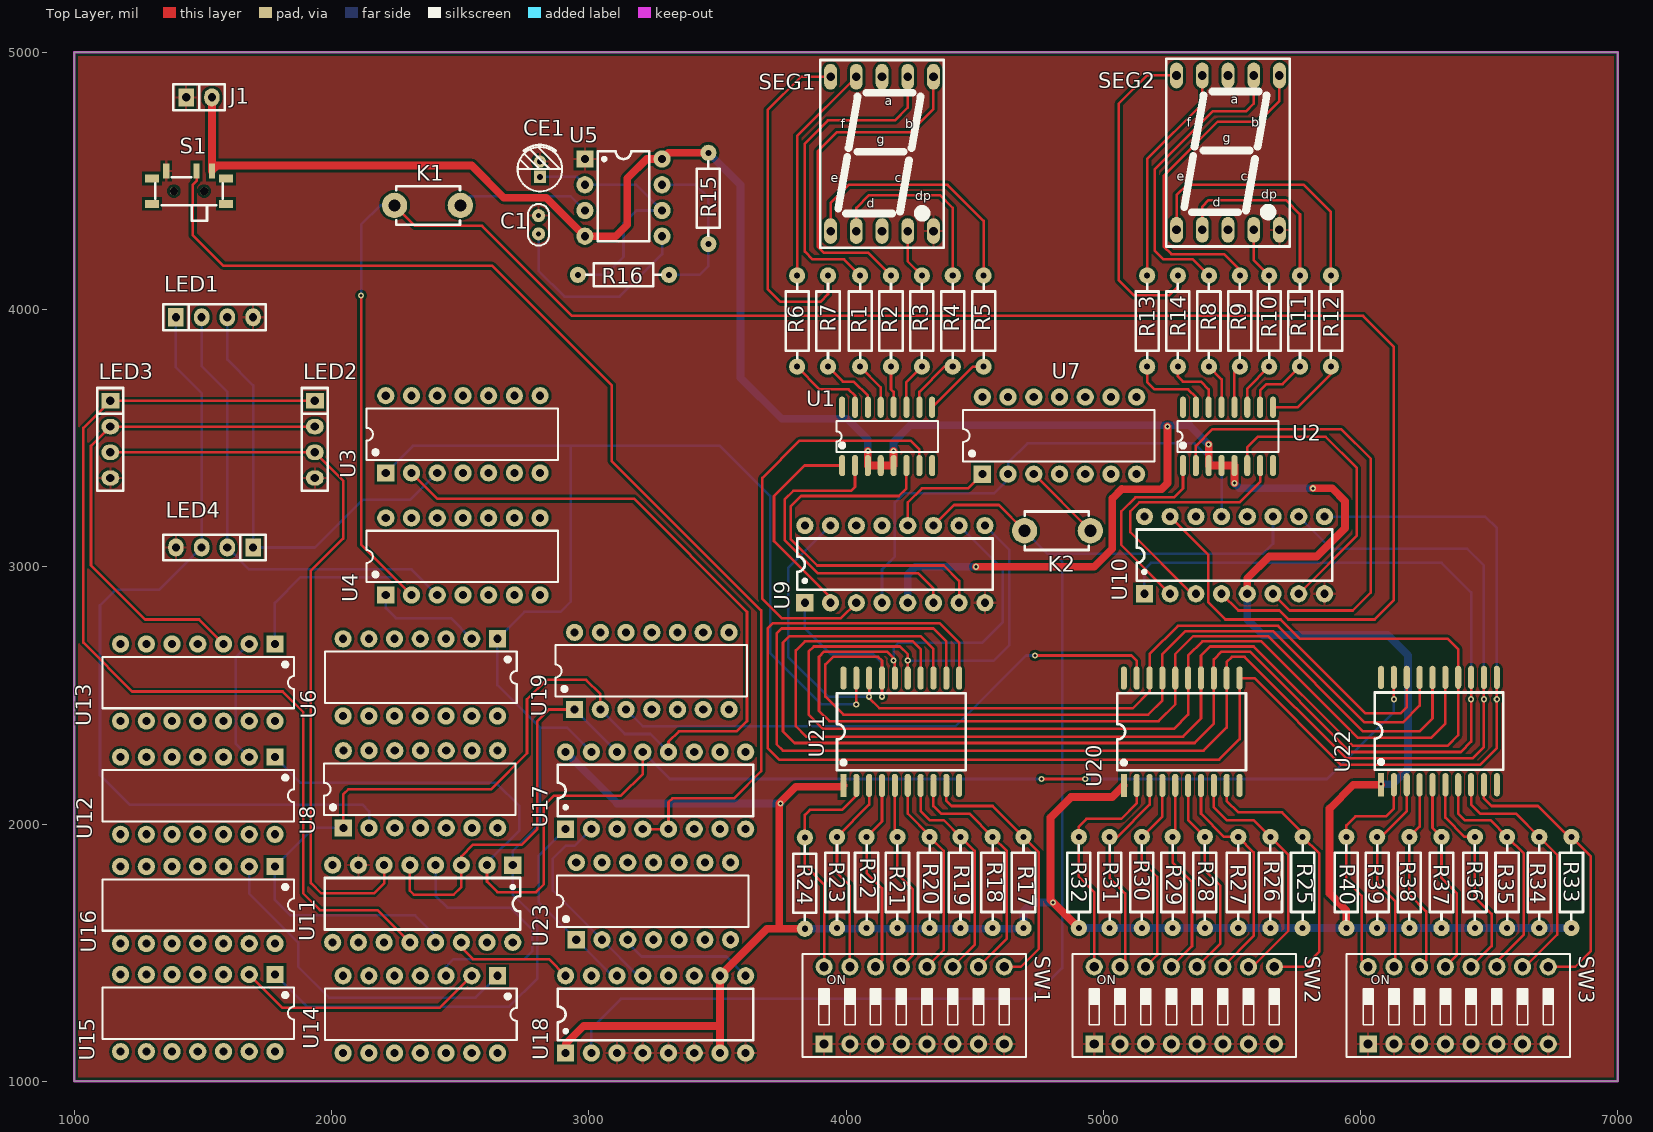
[diagram p0: Top Layer view]
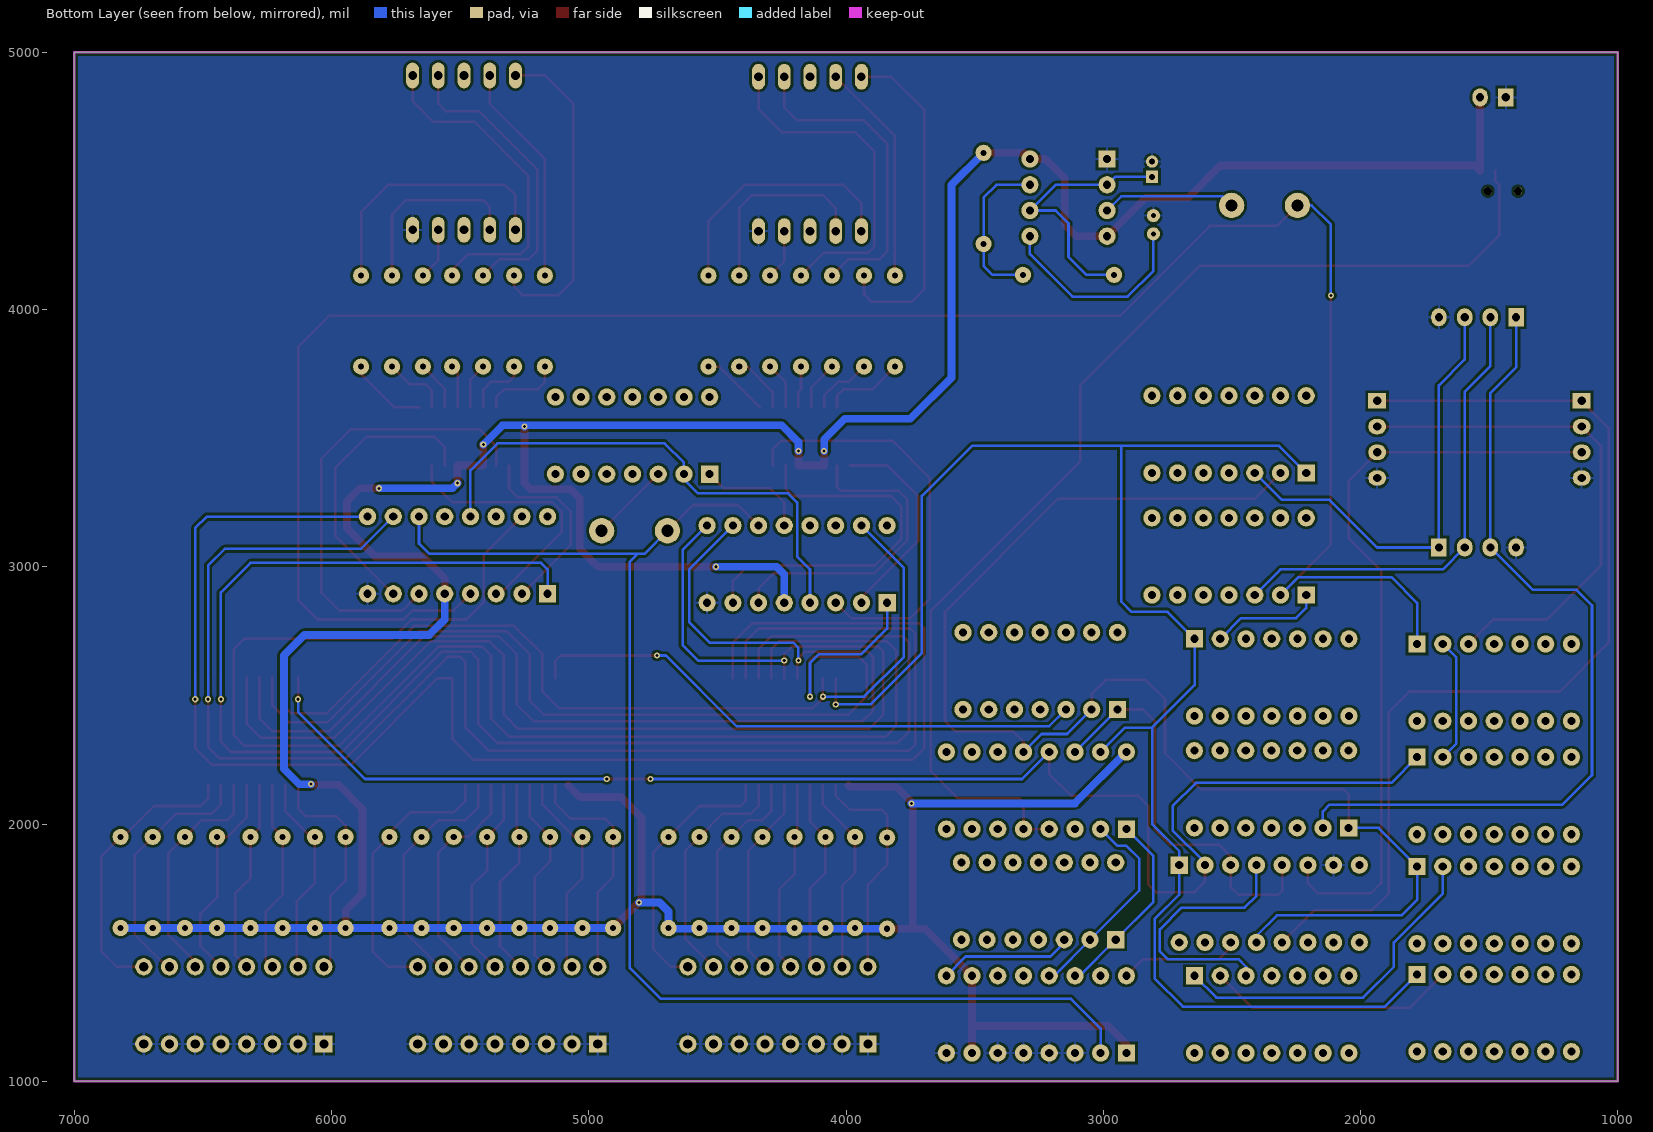
[diagram p1: Bottom Layer view, seen from below]
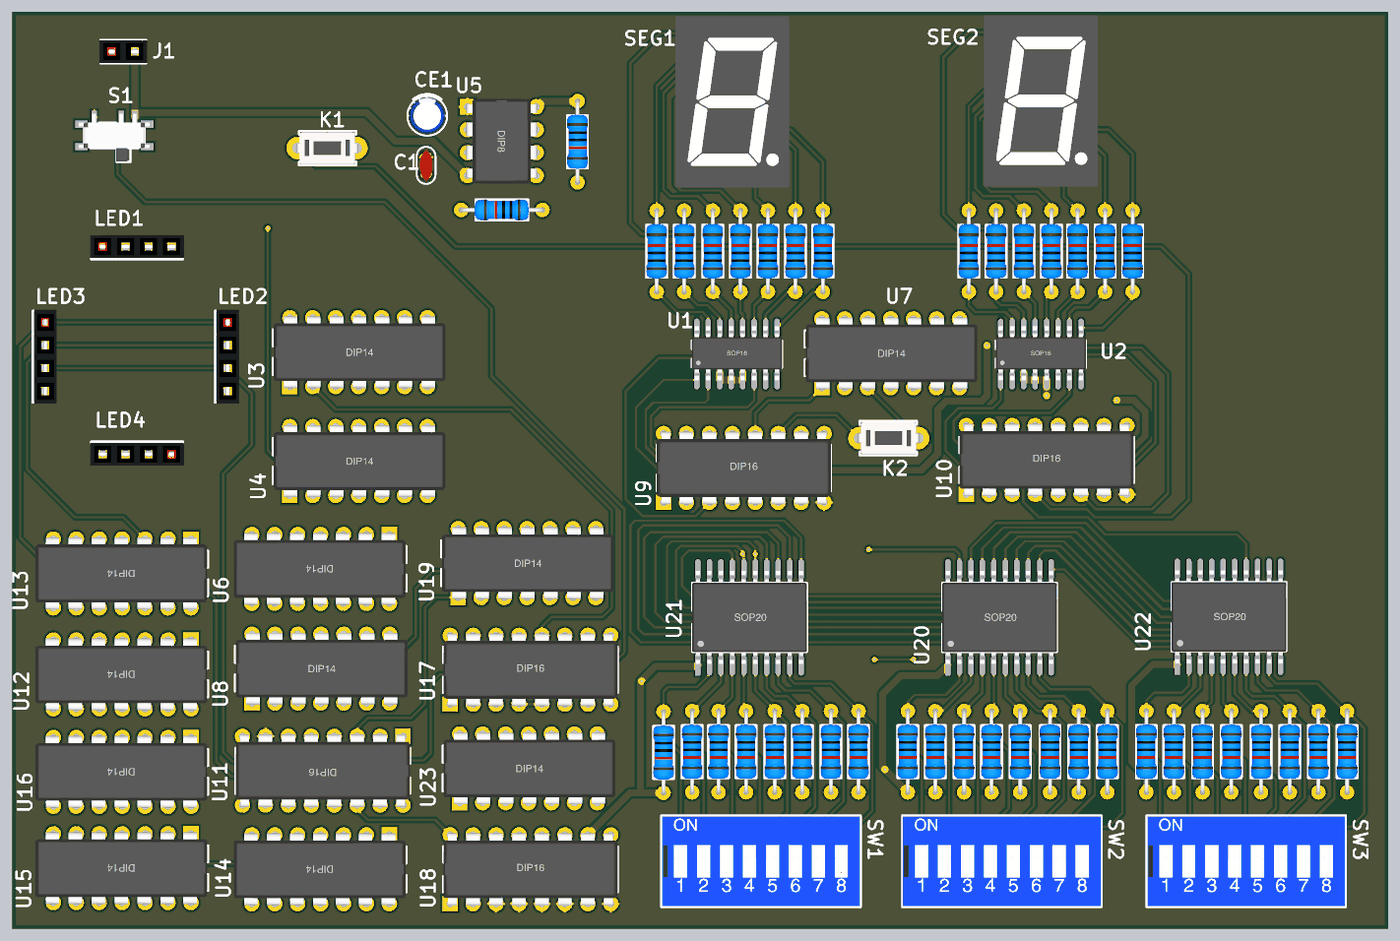
[diagram p2: 3D render of the assembled board from above, using the file's embedded part models]
# Altium PCB MISC82158.PcbDoc
Units mil, origin at the board's own origin, x right, y up, seen from the top; angles counter-clockwise.
Board outline 6000 x 4000 mil, 2 copper layers (Top Layer, Bottom Layer); 78 components, 100 nets, 531 pads, 23 vias.

## Layer stack, top to bottom (the 12.6 mil dielectric is the usual default, probably not edited)
Top Solder: solder mask 0.4, Solder Resist, Dk 3.5
Top Layer: signal copper 1.4
Dielectric 1: dielectric 12.6, FR-4, Dk 4.8
Bottom Layer: signal copper 1.4
Bottom Solder: solder mask 0.4, Solder Resist, Dk 3.5

## Board outline
1000,1000 7000,1000 7000,5000 1000,5000

## Design rules (kind name [scope] priority, off if disabled: settings)
Clearance [All] p1: gap=10
HoleSize [All] p1: absolutevalues=TRUE maxlimit=10000 minlimit=1 maxpercent=80.000 minpercent=20.000
MinimumSolderMaskSliver [All] p1: minsoldermaskwidth=0
PolygonConnect [All] p1: connectstyle=Relief reliefconductorwidth=10 reliefentries=4 polygonreliefangle="90 Angle" airgapwidth=10
RoutingVias [All] p1: holewidth=28 width=50 viastyle="Through Hole" minholewidth=28 minwidth=50 maxholewidth=28 maxwidth=50
SilkToSilkClearance [All] p1: silktosilkclearance=0
SilkToSolderMaskClearance [IsPad] p1: minsilkscreentomaskgap=0 clearancetoexposedcopper=TRUE
SolderMaskExpansion [All] p1: expansion=4
Width [All] p1: maxlimit=100 minlimit=10 preferedwidth=10
26 further rules are at their usual default settings.

## Components (designator, comment, footprint, x,y, rotation, side; value= is the part's Value field where it differs from the comment)
C1 "10nF" "CC 1.8*3.6" 2805,4329.57 r270 top
CE1 "10uF" "CAP 1.5*4*8" 2810,4545.47 r90 top
J1 "Female HDR1X2" Fe-HDR1X2/2.54-S 1435,4825 r0 top
K1 "KEY" DIP-3X6X4.3 2245,4405 r0 top
K2 "KEY" DIP-3X6X4.3 4950,3140 r180 top
LED1 "RGB-3528" Fe-HDR1X4/2.54-S 1395,3970 r90 top
LED2 "RGB-3528" Fe-HDR1X4/2.54-S 1935,3645 r0 top
LED3 "RGB-3528" Fe-HDR1X4/2.54-S 1140,3645 r0 top
LED4 "RGB-3528" Fe-HDR1X4/2.54-S 1695,3075 r270 top
R1 "200" "RS 1/4W" 4055,3955 r90 top
R2 "200" "RS 1/4W" 4175,3955 r90 top
R3 "200" "RS 1/4W" 4295,3955 r90 top
R4 "200" "RS 1/4W" 4415,3955 r90 top
R5 "200" "RS 1/4W" 4535,3955 r90 top
R6 "200" "RS 1/4W" 3810,3955 r90 top
R7 "200" "RS 1/4W" 3930,3955 r90 top
R8 "200" "RS 1/4W" 5410.92,3955 r90 top
R9 "200" "RS 1/4W" 5530.92,3955 r90 top
R10 "200" "RS 1/4W" 5645,3955 r90 top
R11 "200" "RS 1/4W" 5765,3955 r90 top
R12 "200" "RS 1/4W" 5885,3955 r90 top
R13 "200" "RS 1/4W" 5170.92,3955 r90 top
R14 "200" "RS 1/4W" 5290,3955 r90 top
R15 "48K" "RS 1/4W" 3465,4432.17 r270 top
R16 "48K" "RS 1/4W" 3135,4135 r180 top
R17 "200" "RS 1/4W" 4690,1772.83 r270 top
R18 "200" "RS 1/4W" 4570,1772.83 r270 top
R19 "200" "RS 1/4W" 4445,1772.83 r270 top
R20 "200" "RS 1/4W" 4325,1772.83 r270 top
R21 "200" "RS 1/4W" 4200,1772.83 r270 top
R22 "200" "RS 1/4W" 4080,1772.83 r270 top
R23 "200" "RS 1/4W" 3965,1772.83 r270 top
R24 "200" "RS 1/4W" 3840,1770 r270 top
R25 "200" "RS 1/4W" 5775,1772.83 r270 top
R26 "200" "RS 1/4W" 5650,1772.83 r270 top
R27 "200" "RS 1/4W" 5525,1772.83 r270 top
R28 "200" "RS 1/4W" 5395,1772.83 r270 top
R29 "200" "RS 1/4W" 5270,1772.83 r270 top
R30 "200" "RS 1/4W" 5150,1772.83 r270 top
R31 "200" "RS 1/4W" 5025,1772.83 r270 top
R32 "200" "RS 1/4W" 4905,1772.83 r270 top
R33 "200" "RS 1/4W" 6820,1772.83 r270 top
R34 "200" "RS 1/4W" 6695,1772.83 r270 top
R35 "200" "RS 1/4W" 6570,1772.83 r270 top
R36 "200" "RS 1/4W" 6445,1772.83 r270 top
R37 "200" "RS 1/4W" 6315,1772.83 r270 top
R38 "200" "RS 1/4W" 6190,1772.83 r270 top
R39 "200" "RS 1/4W" 6065,1772.83 r270 top
R40 "200" "RS 1/4W" 5945,1772.83 r270 top
S1 "SS-12F23" MSK-12C01-07 1445.94,4460 r0 top
SEG1 "0.56IN-1-A" 0.56IN-1P 3940,4305 r0 top
SEG2 "0.56IN-1-A" 0.56IN-1P 5285,4310 r0 top
SW1 "SW-8P" "CSW DIP-8P" 4265,1295 r0 top
SW2 "SW-8P" "CSW DIP-8P" 5315,1295 r0 top
SW3 "SW-8P" "CSW DIP-8P" 6380,1295 r0 top
U1 "SN74LS48D" SOP16 3985,3393.62 r90 top
U2 "SN74LS48D" SOP16 5310,3393.62 r90 top
U3 "74LS08" DIP14 2510.91,3515 r90 top
U4 "74LS08" DIP14 2510.91,3040 r90 top
U5 "NE555P" DIP8 3135,4435 r0 top
U6 "74LS04" DIP14 2345,2570 r270 top
U7 "74LS32" DIP14 4830,3510 r90 top
U8 "74LS04" DIP14 2345.91,2135 r90 top
U9 "DM74LS192N" DIP16 4190,3010 r90 top
U10 "DM74LS192N" DIP16 5510,3045 r90 top
U11 "DM74ALS11AM" DIP16 2354.43,1690 r270 top
U12 "74LS04" DIP14 1480,2110 r270 top
U13 "74LS08" DIP14 1480,2550 r270 top
U14 "74LS32" DIP14 2345,1260 r270 top
U15 "74LS04" DIP14 1480,1265 r270 top
U16 "74LS04" DIP14 1480,1685 r270 top
U17 "SN74LS138N" DIP16 3260,2130 r90 top
U18 "SN74LS161D" DIP16 3260,1260 r90 top
U19 "74LS08" DIP14 3245,2595 r90 top
U20 "SN74LS245DW" SOP20 5080,2150 r90 top
U21 "SN74LS245DW" SOP20 3990,2150 r90 top
U22 "SN74LS245DW" SOP20 6080,2152.68 r90 top
U23 "74LS00" DIP14 3251.47,1700 r90 top

## Footprints (in the part's own frame and the unit in brackets; to place one, negate y for a bottom-side part, rotate by r counter-clockwise, add the part's x,y. Pads: shape width x height; smd on the part's side, far side on the other; paste and mask are expansions set on the pad)
0.56IN-1P [mm]
  oval 1.27x2.54 hole 0.85: 1(0,0) 2(2.54,0) 3(5.08,0) 4(7.62,0) 5(10.16,0) 6(10.16,15.24) 7(7.62,15.24) 8(5.08,15.24) 9(2.54,15.24) 10(0,15.24)
  silkscreen extent -1.02,-1.65 11.18,16.89, body extent -1.22,-1.85 11.38,17.14, height 8
"CAP 1.5*4*8" [mm] "脚距1.5mm直径4mm高度8mm"
  rect 1.2x1.2 hole 0.6: 1(-0.75,0)
  round 1.2 hole 0.6: 2(0.75,0)
  silkscreen extent -2.2,-2.2 2.41,2.2, body extent -2,-2 2.02,2, height 8.04
"CC 1.8*3.6" [mm] "脚距1.8mm直径3.6mm"
  round 1.3 hole 0.5: 1(-0.9,0) 2(0.9,0)
  silkscreen extent -2.05,-1.04 2.05,1.04, body extent -1.8,-0.8 1.8,0.8, height 3.6
"CSW DIP-8P" [mm] "21.9*9.9*7mm"
  rect 1.7x1.7 hole 0.9: 1(-8.89,-3.81)
  round 1.7 hole 0.9: 2(-6.35,-3.81) 3(-3.81,-3.81) 4(-1.27,-3.81) 5(1.27,-3.81) 6(3.81,-3.81) 7(6.35,-3.81) 8(8.89,-3.81) 9(8.89,3.81) 10(6.35,3.81) 11(3.81,3.81) 12(1.27,3.81) 13(-1.27,3.81) 14(-3.81,3.81) 15(-6.35,3.81) 16(-8.89,3.81)
  silkscreen extent -11.05,-5.08 11.05,5.08, body extent -10.94,-4.95 10.94,4.95, height 6.65
DIP8 [mm]
  rect 1.7x1.7 hole 0.8: 1(-3.81,3.81)
  round 1.7 hole 0.8: 2(-3.81,1.27) 3(-3.81,-1.27) 4(-3.81,-3.81) 5(3.81,-3.81) 6(3.81,-1.27) 7(3.81,1.27) 8(3.81,3.81)
  silkscreen extent -2.54,-4.32 2.54,4.57, body extent -3.94,-4.7 3.91,4.7, height 4.5
DIP14 [mm]
  rect 1.7x1.7 hole 0.8: 1(-3.81,7.62)
  round 1.7 hole 0.8: 2(-3.81,5.08) 3(-3.81,2.54) 4(-3.81,0) 5(-3.81,-2.54) 6(-3.81,-5.08) 7(-3.81,-7.62) 8(3.81,-7.62) 9(3.81,-5.08) 10(3.81,-2.54) 11(3.81,0) 12(3.81,2.54) 13(3.81,5.08) 14(3.81,7.62)
  silkscreen extent -2.54,-9.4 2.54,9.53, body extent -3.98,-9.6 3.98,9.4, height 4.1
DIP16 [mm]
  rect 1.7x1.7 hole 0.8: 1(-3.81,8.89)
  round 1.7 hole 0.8: 2(-3.81,6.35) 3(-3.81,3.81) 4(-3.81,1.27) 5(-3.81,-1.27) 6(-3.81,-3.81) 7(-3.81,-6.35) 8(-3.81,-8.89) 9(3.81,-8.89) 10(3.81,-6.35) 11(3.81,-3.81) 12(3.81,-1.27) 13(3.81,1.27) 14(3.81,3.81) 15(3.81,6.35) 16(3.81,8.89)
  silkscreen extent -2.54,-9.65 2.54,9.65, body extent -4.02,-9.65 4.02,9.65, height 4.45
DIP-3X6X4.3 [mm]
  round 2.5 hole 1.2: 1(0,0) 3(6.5,0)
  silkscreen extent 0.16,-1.9 6.46,1.9, body extent -0.64,-1.75 7.19,1.75, height 4.31
Fe-HDR1X2/2.54-S [mil] "Connector; Header; 2x2 Position"
  rect 60x70 hole 32: 1(0,0)
  oval 60x70 hole 32: 2(100,0)
  silkscreen extent -50,-50 150,50, body extent -55,-48 155,50, height 335
Fe-HDR1X4/2.54-S [mil]
  rect 70x60 hole 32: 1(0,0)
  oval 70x60 hole 32: 2(0,-100) 3(0,-200) 4(0,-300)
  silkscreen extent -50,-350 50,50, body extent -44,-355 54,55, height 335
MSK-12C01-07 [mm] "6.7*2.8*1.5mm(长宽高）"
  rect 1.4x0.8 smd: 0(-3.65,-1.25) 0(-3.65,1.25) 0(3.65,-1.25) 0(3.65,1.25)
  rect 0.6x1.5 smd: 1(-2.25,1.996) 2(0.75,1.996) 3(2.25,1.996)
  round 0.8 hole 0.8: " "(-1.5,0) " "(1.5,0)
  silkscreen extent -3.35,-2.92 3.35,1.4, body extent -3.92,-2.9 3.92,2.4, height 1.5
"RS 1/4W" [mm] "直插色环电阻，脚距9mm，直径2.3mm"
  round 1.6 hole 0.6: 1(-4.5,0) 2(4.5,0)
  silkscreen extent -3.68,-1.14 3.68,1.14, body extent -4.72,-1.16 4.73,1.16, height 2.32
SOP16 [mm]
  oval 2.1x0.6 smd: 1(0,0) 2(0,-1.27) 3(0,-2.54) 4(0,-3.81) 5(0,-5.08) 6(0,-6.35) 7(0,-7.62) 8(0,-8.89) 9(5.75,-8.89) 10(5.75,-7.62) 11(5.75,-6.35) 12(5.75,-5.08) 13(5.75,-3.81) 14(5.75,-2.54) 15(5.75,-1.27) 16(5.75,0)
  silkscreen extent 1.35,-9.45 4.4,0.56, body extent -0.04,-9.45 5.97,0.56, height 1.9
SOP20 [mm]
  rect 2.3x0.6 smd: 1(0,0)
  oval 2.3x0.6 smd: 2(0,-1.27) 3(0,-2.54) 4(0,-3.81) 5(0,-5.08) 6(0,-6.35) 7(0,-7.62) 8(0,-8.89) 9(0,-10.16) 10(0,-11.43) 11(10.6,-11.43) 12(10.6,-10.16) 13(10.6,-8.89) 14(10.6,-7.62) 15(10.6,-6.35) 16(10.6,-5.08) 17(10.6,-3.81) 18(10.6,-2.54) 19(10.6,-1.27) 20(10.6,0)
  silkscreen extent 1.49,-12.06 9.11,0.64, body extent 0.13,-12.06 10.44,0.64, height 2.7

## Part data
C1: library part CC, "Ceramic capacitor"
CE1: library part CE, "Through-hole electrolytic capacitor"
LED1 LED2 LED3 LED4: library part "LED-RGB 3528", "3528 RGB LED"
R1 R2 R3 R4 R5 R6 R7 R8 R9 R10 R11 R12 R13 R14 R15 R16 R17 R18 R19 R20 R21 R22 R23 R24 R25 R26 R27 R28 R29 R30 R31 R32 R33 R34 R35 R36 R37 R38 R39 R40: library part R-S, "Color-band resistor"
S1: library part SSW-1P, "1-way wave switch"
SEG1 SEG2: "1-digit 0.56 inch common-anode display"
SW1 SW2 SW3: "8-way coded switch"
U1 U2: "BCD-to-Seven-Segment Decoder/Driver"
U3 U4 U13 U19: "Quad 2-input AND gate"
U5: "Precision Timer"
U6 U8 U12 U15 U16: "Hex inverter"
U7 U14: "Quad 2-input OR gate"
U9 U10: "Up/Down Decade Counter with Separate Up/Down Clock"
U11: "Triple 3-Input AND Gate"
U17: "1-of-8 Decoder/Demultiplexer"
U18: library part SN74LS161A, "SYN 4-BIT CNT"
U20 U21 U22: "Octal Bus Transceiver"
U23: "Quad 2-input NAND gate"

## Via types
v1: diameter 24, hole 12, Top Layer to Bottom Layer, 23 vias

## Nets (pads, with @x,y where several pads share a name; then routed paths per layer and width w, separated by ;. In a path a pad name is that pad's centre, name@x,y a point inside that pad or via, vN(x,y) a via of type N, cw(c..) or ccw(c..) an arc to the next point about the centre after c; other vN are vias at no path point)
+5V: J1.2 R15.1 R17.2 R18.2 R19.2 R20.2 R21.2 R22.2 R23.2 R24.2 R25.2 R26.2 R27.2 R28.2 R29.2 R30.2 R31.2 R32.2 R33.2 R34.2 R35.2 R36.2 R37.2 R38.2 R39.2 R40.2 S1.3 U1.3 U1.4 U1.5 U2.3 U2.4 U2.5 U5.4 U5.8 U9.5 U10.5 U17.16 U18.1 U18.7 U18.10 U20.1 U21.1 U22.1 | length 17510.7
  Top Layer w30: S1.3 S1.3@1535,4539.06 ; J1.2 S1.3@1535,4539.06 ; U18.1 2910,1145 2980,1215 3510,1215 ; R15.1 3309.33,4609.33 U5.8 3225,4585 3150,4510 3150,4330 3105,4285 U5.4 2835,4435 2670,4435 2545,4560 1555.94,4560 S1.3@1535,4539.06 ; U18.7 3510,1215 ; R24.2 3740,1592.83 ; U21.1 3985,2145 3805,2145 3740,2080 3740,1592.83 ; v1(4085,3450) U1.3 U1.4 4168.62,3393.62 ; U1.5 v1(4185,3450) ; v1(4505,3000) 4965,3000 5035,3070 5035,3265 5072.5,3302.5 5073.46,3301.54 5226.54,3301.54 5250,3325 v1(5250,3545) ; R32.2 4795,1705.67 4795,2025 4875,2105 5035,2105 U20.1 ; v1(5410,3475) U2.3 U2.4 U2.5 v1(5510,3325) ; U10.5 5560,2955 5645,3040 5830,3040 5940,3150 5940,3255 5890,3305 v1(5815,3305) ; R40.2 5945,1665 5880,1730 5880,2060 5972.68,2152.68 U22.1 ; 3510,1215 U18.10 3692.83,1592.83 3740,1592.83
  Bottom Layer w30: U17.16 3110,2080 v1(3745,2080) ; R15.1 3590,4484.33 3590,3735 3750,3575 4005,3575 4085,3495 v1(4085,3450) ; R24.2 4687.17,1592.83 R17.2 4690,1660 4725,1695 v1(4805,1695) ; v1(4185,3450) 4185,3485 4250,3550 v1@5255,3550 ; U9.5 4240,2970 4270,3000 v1(4505,3000) ; R32.2 R31.2 R30.2 R29.2 R28.2 R27.2 R26.2 R25.2 R40.2 R39.2 R38.2 R37.2 R36.2 R35.2 R34.2 R33.2 ; v1(5250,3545) v1@5255,3550 ; v1(5410,3475) 5335,3550 v1@5255,3550 ; v1(5510,3325) 5530,3305 v1(5815,3305) ; U10.5 5560,2795 5620,2735 6105,2735 6185,2655 6185,2215 6125,2155 v1(6080,2155)
GND: C1.1 CE1.2 J1.1 LED1.4 LED2.4 LED3.4 LED4.4 S1.1 SEG1.5 SEG2.5 SW1.1 SW1.2 SW1.3 SW1.4 SW1.5 SW1.6 SW1.7 SW1.8 SW2.1 SW2.2 SW2.3 SW2.4 SW2.5 SW2.6 SW2.7 SW2.8 SW3.1 SW3.2 SW3.3 SW3.4 SW3.5 SW3.6 SW3.7 SW3.8 U5.1 U9.8 U10.8 U11.7 U18.3 U18.4 U18.5 U18.6 U18.8
NetC1_2: C1.2 U5.5 | length 803.9
  Bottom Layer w10: C1.2 2805,4150 2905,4050 3120,4050 3285,4215 U5.5
NetCE1_1: CE1.1 R16.2 U5.2 U5.6 | length 1036.1
  Bottom Layer w10: CE1.1 2954.06,4515.94 U5.2 3185,4485 U5.6 3185,4385 3135,4335 3135,4205 3065,4135 R16.2
NetK1_1: K1.1 U4.2 U10.4 U13.1 | length 8283.8
  Top Layer w10: v1(2115,4055) 2115,3085.91 U4.2 ; K1.1 2325,4325 2585,4325 2935,3975 6010,3975 6130,3855 6130,2870 6055,2795 5720,2795 5685,2830 5525,2830 U10.4
  Bottom Layer w10: U13.1 1780,2860 1880,2960 2240.91,2960 U4.2 ; v1(2115,4055) 2115,4330 2190,4405 K1.1
NetK1_3: K1.3 U5.3 | length 521.4
  Bottom Layer w10: K1.3 2535.91,4440 2930,4440 U5.3
NetK2_1: K2.1 U7.3 | length 311.1
  Top Layer w10: U7.3 K2.1
NetK2_3: K2.3 U9.11 U10.11 U18.2 | length 5203.2
  Top Layer w10: U9.11 4420,3240 4594.09,3240 K2.3 ; U10.11@5655,3195 U10.11
  Bottom Layer w10: U18.2 3010,1205 3125,1320 4720,1320 4840,1440 4840,3020 4810,3050 ; K2.3 4784.09,3050 4810,3050 ; U10.11 5660,3090 5620,3050 4810,3050
NetLED1_1: LED1.1 LED4.3 U8.2 | length 3253
  Bottom Layer w10: LED1.1 1395,3775 1495,3675 LED4.3 1330,2910 1160,2910 1100,2850 1100,2190 1215,2075 2120,2075 2145.91,2049.09 U8.2
NetLED1_2: LED1.2 LED4.2 U4.3 | length 1829
  Bottom Layer w10: LED1.2 1495,3780 1595,3680 LED4.2 1680,2990 2310.91,2990 U4.3
NetLED1_3: LED1.3 LED4.1 U3.3 | length 1772.4
  Bottom Layer w10: LED1.3 1595,3805 1695,3705 LED4.1 1935,3075 2120,3260 2305.91,3260 U3.3
NetLED2_1: LED2.1 LED3.1 U11.12 | length 3943.5
  Top Layer w10: LED2.1 LED3.1 1035,3540 1035,2705 1225,2515 1810,2515 1890,2435 1890,1730 1955,1665 2179.43,1665 U11.12
NetLED2_2: LED2.2 LED3.2 U13.3 | length 2007.4
  Top Layer w10: U13.3 1485,2795 1275,2795 1065,3005 1065,3470 LED3.2 LED2.2
NetLED2_3: LED2.3 LED3.3 U11.6 | length 2955.2
  Top Layer w10: LED3.3 LED2.3 2045,3335 2045,3110 1920,2985 1920,1770 1960,1730 2165,1730 2204.43,1769.43 U11.6
NetR1_1: R1.1 U1.13 | length 191
  Top Layer w10: R1.1 4135,3697.83 U1.13
NetR1_2: R1.2 SEG1.7 | length 1251.4
  Top Layer w10: R1.2 3992.17,4195 3870,4195 3840,4225 3840,4645 3930,4735 4190,4735 4240,4785 SEG1.7
NetR2_1: R2.1 U1.12 | length 162
  Top Layer w10: R2.1 4175,3690 4185,3680 U1.12
NetR2_2: R2.2 SEG1.6 | length 1345.1
  Top Layer w10: R2.2 4087.17,4220 3915,4220 3890,4245 3890,4615 3965,4690 4250,4690 4340,4780 SEG1.6
NetR3_1: R3.1 U1.11 | length 182.7
  Top Layer w10: U1.11 4235,3717.83 R3.1
NetR3_2: R3.2 SEG1.4 | length 195.6
  Top Layer w10: SEG1.4 4240,4187.17 R3.2
NetR4_1: R4.1 U1.10 | length 230.5
  Top Layer w10: U1.10 4285,3680 4382.83,3777.83 R4.1
NetR4_2: R4.2 SEG1.2 | length 769.3
  Top Layer w10: SEG1.2 4040,4395 4090,4445 4365,4445 4415,4395 R4.2
NetR5_1: R5.1 U1.9 | length 265.4
  Top Layer w10: U1.9 4492.83,3777.83 R5.1
NetR5_2: R5.2 SEG1.1 | length 1004.8
  Top Layer w10: SEG1.1 3940,4415 4010,4485 4395,4485 4535,4345 R5.2
NetR6_1: R6.1 U1.15 | length 316.7
  Top Layer w10: R6.1 3897.83,3690 4010,3690 4035,3665 U1.15
NetR6_2: R6.2 SEG1.9 | length 868.1
  Top Layer w10: R6.2 3810,4675 SEG1.9
NetR7_1: R7.1 U1.14 | length 246.7
  Top Layer w10: R7.1 3987.83,3720 4030,3720 4085,3665 U1.14
NetR7_2: R7.2 SEG1.10 | length 1334.2
  Top Layer w10: R7.2 3930,4060 3900,4030 3745,4030 3695,4080 3695,4775 3825,4905 SEG1.10
NetR8_1: R8.1 U2.13 | length 178.2
  Top Layer w10: R8.1 5460,3728.76 U2.13
NetR8_2: R8.2 SEG2.7 | length 1167.1
  Top Layer w10: R8.2 5348.09,4195 5235,4195 5200,4230 5200,4545 5425,4770 5555,4770 5585,4800 SEG2.7
NetR9_1: R9.1 U2.12 | length 166.5
  Top Layer w10: U2.12 5510,3756.91 R9.1
NetR9_2: R9.2 SEG2.6 | length 1300.6
  Top Layer w10: R9.2 5530.92,4154.08 5470,4215 5265,4215 5235,4245 5235,4520 5445,4730 5605,4730 5685,4810 SEG2.6
NetR10_1: R10.1 U2.11 | length 193
  Top Layer w10: U2.11 5560,3692.83 R10.1
NetR10_2: R10.2 SEG2.4 | length 202.7
  Top Layer w10: SEG2.4 5585,4192.17 R10.2
NetR11_1: R11.1 U2.10 | length 258.5
  Top Layer w10: U2.10 5610,3685 5635,3710 5697.17,3710 R11.1
NetR11_2: R11.2 SEG2.2 | length 741
  Top Layer w10: SEG2.2 5385,4400 5410,4425 5710,4425 5765,4370 R11.2
NetR12_1: R12.1 U2.9 | length 306.7
  Top Layer w10: U2.9 5755,3620 5885,3750 R12.1
NetR12_2: R12.2 SEG2.1 | length 1042.9
  Top Layer w10: SEG2.1 5285,4445 5325,4485 5780,4485 5885,4380 R12.2
NetR13_1: R13.1 U2.15 | length 312.3
  Top Layer w10: R13.1 5170.92,3719.08 5200,3690 5330,3690 5360,3660 U2.15
NetR13_2: R13.2 SEG2.9 | length 866.5
  Top Layer w10: R13.2 5170.92,4585.92 5385,4800 SEG2.9
NetR14_1: R14.1 U2.14 | length 248.5
  Top Layer w10: R14.1 5290,3740 5310,3720 5380,3720 5410,3690 U2.14
NetR14_2: R14.2 SEG2.10 | length 1267.1
  Top Layer w10: SEG2.10 5170,4910 5060,4800 5060,4115 5120,4055 5255,4055 5290,4090 R14.2
NetR15_2: R15.2 R16.1 U5.7 | length 633
  Bottom Layer w10: U5.7 3415,4485 3465,4435 R15.2 3465,4170 3430,4135 R16.1
NetR17_1: R17.1 SW1.9 U21.9 | length 1041.8
  Top Layer w10: U21.9 4390,2090 4410,2070 4570,2070 R17.1 4750,1890 4750,1515 4680,1445 SW1.9
NetR18_1: R18.1 SW1.10 U21.8 | length 933.1
  Top Layer w10: U21.8 4340,2070 4370,2040 4480,2040 R18.1 4625,1895 4625,1555 SW1.10
NetR19_1: R19.1 SW1.11 U21.7 | length 859.4
  Top Layer w10: U21.7 4290,2050 4325,2015 4380,2015 R19.1 4500,1895 4500,1530 SW1.11
NetR20_1: R20.1 SW1.12 U21.6 | length 789.9
  Top Layer w10: U21.6 4240,2040 4325,1955 R20.1 4380,1895 4380,1510 SW1.12
NetR21_1: R21.1 SW1.13 U21.5 | length 752.6
  Top Layer w10: U21.5 4190,1960 R21.1 4200,1805 4260,1745 4260,1490 SW1.13
NetR22_1: R22.1 SW1.14 U21.4 | length 765.1
  Top Layer w10: SW1.14 4140,1470 4140,1750 4080,1810 R22.1 4140,2010 U21.4
NetR23_1: R23.1 SW1.15 U21.3 | length 777.5
  Top Layer w10: SW1.15 4015,1760 3965,1810 R23.1 4090,2075 U21.3
NetR24_1: R24.1 SW1.16 U21.2 | length 892.1
  Top Layer w10: SW1.16 3915,1765 3840,1840 R24.1 3840,2035 3860,2055 3985,2055 4040,2110 U21.2
NetR25_1: R25.1 SW2.9 U20.9 | length 1093.6
  Top Layer w10: U20.9 5480,2090 5525,2045 5695,2045 5775,1965 R25.1 5840,1885 5840,1505 5780,1445 SW2.9
NetR26_1: R26.1 SW2.10 U20.8 | length 959.6
  Top Layer w10: U20.8 5430,2065 5480,2015 5585,2015 R26.1 5720,1880 5720,1585 5580,1445 SW2.10
NetR27_1: R27.1 SW2.11 U20.7 | length 871.8
  Top Layer w10: U20.7 5380,2040 5470,1950 R27.1 5585,1890 5585,1565 SW2.11
NetR28_1: R28.1 SW2.12 U20.6 | length 794.1
  Top Layer w10: U20.6 5330,2015 R28.1 5395,1820 5455,1760 5455,1535 SW2.12
NetR29_1: R29.1 SW2.13 U20.5 | length 773.3
  Top Layer w10: SW2.13 5345,1525 5345,1775 5270,1850 R29.1 5280,1960 U20.5
NetR30_1: R30.1 SW2.14 U20.4 | length 781.6
  Top Layer w10: SW2.14 5210,1490 5210,1795 5150,1855 R30.1 5230,2030 U20.4
NetR31_1: R31.1 SW2.15 U20.3 | length 819.9
  Top Layer w10: SW2.15 5085,1465 5085,1730 5025,1790 R31.1 5055,1950 5180,2075 U20.3
NetR32_1: R32.1 SW2.16 U20.2 | length 902.1
  Top Layer w10: SW2.16 4965,1735 4905,1795 R32.1 4905,1990 4935,2020 5070,2020 5130,2080 U20.2
NetR33_1: R33.1 SW3.9 U22.9 | length 1120.7
  Top Layer w10: U22.9 6480,2100 6510,2070 6690,2070 6810,1950 R33.1 6895,1875 6895,1505 6835,1445 SW3.9
NetR34_1: R34.1 SW3.10 U22.8 | length 990.2
  Top Layer w10: U22.8 6430,2075 6465,2040 6605,2040 R34.1 6765,1880 6765,1570 6640,1445 SW3.10
NetR35_1: R35.1 SW3.11 U22.7 | length 915.4
  Top Layer w10: U22.7 6380,2040 6405,2015 6505,2015 R35.1 6635,1885 6635,1570 6530,1465 SW3.11
NetR36_1: R36.1 SW3.12 U22.6 | length 838.8
  Top Layer w10: U22.6 6330,2025 6405,1950 R36.1 6445,1715 6510,1650 6510,1525 SW3.12
NetR37_1: R37.1 SW3.13 U22.5 | length 765.7
  Top Layer w10: U22.5 6280,1985 R37.1 6315,1790 6375,1730 6375,1490 SW3.13
NetR38_1: R38.1 SW3.14 U22.4 | length 761.5
  Top Layer w10: SW3.14 6255,1470 6255,1660 6190,1725 R38.1 6230,1990 U22.4
NetR39_1: R39.1 SW3.15 U22.3 | length 795.2
  Top Layer w10: SW3.15 6135,1450 6135,1700 6065,1770 R39.1 6080,1950 6180,2050 U22.3
NetR40_1: R40.1 SW3.16 U22.2 | length 889.8
  Top Layer w10: SW3.16 6005,1470 6005,1720 5945,1780 R40.1 5945,1995 5980,2030 6100,2030 6130,2060 U22.2
NetS1_2: S1.2 U17.4 U17.5 | length 4482.3
  Top Layer w10: S1.2 1475.47,4500 1460,4484.53 1460,4290 1580,4170 2625,4170 3090,3705 3090,3410 3670,2830 3670,2205 3565,2100 3325,2100 3310,2085 U17.5 U17.4
NetU1_1: U1.1 U9.2 | length 820.3
  Top Layer w10: U9.2 3940,2880 3720,3100 3720,3275 3838.62,3393.62 U1.1
NetU1_2: U1.2 U9.6 | length 1245.9
  Top Layer w10: U1.2 4035,3310 4020,3295 3795,3295 3762.54,3262.54 3762.54,3102.46 3890,2975 4280,2975 4340,2915 U9.6
NetU1_6: U1.6 U9.7 | length 1502
  Top Layer w10: U1.6 4235,3305 4205,3275 3825,3275 3785,3235 3785,3108.28 3888.28,3005 4380,3005 4440,2945 U9.7
NetU1_7: U1.7 U9.3 | length 1636.9
  Top Layer w10: U9.3 3980,2800 3750,2800 3675,2875 3675,3345 3820,3490 4250,3490 4285,3455 U1.7
NetU2_1: U2.1 U10.2 | length 764.6
  Top Layer w10: U10.2 5070,3085 5070,3215 5125,3270 5275,3270 5310,3305 U2.1
NetU2_2: U2.2 U10.6 | length 1786.9
  Top Layer w10: U2.2 5360,3470 5425,3535 5925,3535 6040,3420 6040,2900 5970,2830 5725,2830 U10.6
NetU2_6: U2.6 U10.7 | length 1145.9
  Top Layer w10: U2.6 5560,3465 5600,3505 5865,3505 5985,3385 5985,3120 U10.7
NetU2_7: U2.7 U10.3 | length 1050.7
  Top Layer w10: U10.3 5345,2895 5105,3135 5105,3215 5140,3250 5530,3250 5610,3330 U2.7
NetU3_1: U3.1 U6.1 U11.1 U15.1 U17.15 U21.19 | length 6526.9
  Top Layer w10: v1(4040,2465) U21.19
  Bottom Layer w10: U15.1 1905,1290 2690,1290 2800,1400 2800,1630 2704.43,1725.57 U11.1 2704.43,1894.43 2810,2000 2810,2375 ; U3.1 2315.91,3470 2930,3470 ; U17.15 2915,2375 2810,2375 ; v1(4040,2465) 3905,2465 3705,2665 3705,3275 3510,3470 2930,3470 ; 2810,2375 2645,2540 U6.1 2750,2825 2890,2825 2930,2865 2930,3470
NetU3_2: U3.2 U8.1 U11.13 U16.1 U17.12 U19.2 | length 5349.8
  Top Layer w10: U8.1 2045.9,2115.91 2065,2135 2620,2135 2760,2275 2760,2485 2835,2560 2990,2560 3045,2505 U19.2 ; U3.2 2410.91,3265 3175,3265 3615,2825 3615,2400 3575,2360 3350,2360 3310,2320 U17.12
  Bottom Layer w10: U8.1 1930,1985 U16.1 1780,1705 1840,1645 2325,1645 2404.43,1565.57 U11.13 ; U19.2 3140,2350 3240,2350 U17.12
NetU4_1: U4.1 U6.2 | length 434.3
  Bottom Layer w10: U4.1 2210.91,2839.09 2250,2800 2465,2800 U6.2
NetU7_1: U7.1 U9.12 | length 425.6
  Top Layer w10: U9.12 4240,3250 4295,3305 4475,3305 U7.1
NetU7_2: U7.2 U9.4 U10.13 | length 2037.5
  Bottom Layer w10: U9.4 4140,2990 4190,3040 4190,3250 4225,3285 4575,3285 4630,3340 U7.2 4630,3405 4705,3480 5355,3480 5460,3375 U10.13
NetU9_1: U9.1 U20.17 U21.17 U22.17 | length 3952.6
  Top Layer w10: v1(4140,2495) U21.17 4140,2635 4125,2650 3950,2650 3920,2620 3920,2495 3990,2425 5175,2425 5230,2480 U20.17 5230,2660 5320,2750 5660,2750 6015,2395 6165,2395 6230,2460 U22.17
  Bottom Layer w10: U9.1 3840,2760 3940,2660 4105,2660 4140,2625 v1(4140,2495)
NetU9_9: U9.9 U20.15 U21.15 U22.15 | length 4799
  Top Layer w10: U21.15 v1(4240,2635) 4240,2660 4210,2690 3875,2690 3855,2670 3855,2425 3910,2370 5275,2370 5330,2425 U20.15 5330,2655 5385,2710 5615,2710 5990,2335 6275,2335 6330,2390 U22.15
  Bottom Layer w10: v1(4240,2635) 4575,2635 4635,2695 4635,3065 U9.9
NetU9_10: U9.10 U20.16 U21.16 U22.16 | length 4546.7
  Top Layer w10: U21.16 4190,2640 4160,2670 3915,2670 3895,2650 3895,2440 3935,2400 5215,2400 5280,2465 U20.16 5280,2660 5350,2730 5640,2730 6010,2360 6230,2360 6280,2410 U22.16
  Bottom Layer w10: v1(4185,2635) 4185,2685 4205,2705 4530,2705 4610,2785 4610,2990 U9.10
NetU9_15: U9.15 U20.18 U21.18 U22.18 | length 3625.1
  Top Layer w10: U21.18 v1(4090,2495) 4090,2490 4130,2450 5115,2450 5180,2515 U20.18 5180,2660 5290,2770 5680,2770 6020,2430 6155,2430 6180,2455 U22.18
  Bottom Layer w10: U9.15 3775,2995 3775,2650 3930,2495 v1(4090,2495)
NetU10_1: U10.1 U20.13 U21.13 U22.13 | length 6327
  Top Layer w10: U21.13 4340,2680 4290,2730 3780,2730 3755,2705 3755,2360 3800,2315 5355,2315 5430,2390 U20.13 5430,2640 5460,2670 5570,2670 5960,2280 6390,2280 6430,2320 v1(6430,2485) U22.13
  Bottom Layer w10: U10.1 5160,2990 5185,3015 6315,3015 6430,2900 v1(6430,2485)
NetU10_9: U10.9 U20.11 U21.11 U22.11 | length 6306.4
  Top Layer w10: U21.11 4440,2705 4365,2780 3715,2780 3695,2760 3695,2295 3740,2250 5450,2250 5530,2330 U20.11 5587.68,2567.32 5925,2230 6465,2230 6530,2295 v1(6530,2485) U22.11
  Bottom Layer w10: U10.9 6485,3195 6530,3150 v1(6530,2485)
NetU10_10: U10.10 U20.12 U21.12 U22.12 | length 6093.5
  Top Layer w10: U21.12 4390,2710 4340,2760 3750,2760 3730,2740 3730,2310 3755,2285 5390,2285 5480,2375 U20.12 5480,2630 5500,2650 5550,2650 5945,2255 6435,2255 6480,2300 v1(6480,2485) U22.12
  Bottom Layer w10: U10.10 5885,3070 6415,3070 6480,3005 v1(6480,2485)
NetU10_15: U10.15 U20.14 U21.14 U22.14 | length 5752.4
  Top Layer w10: U21.14 4290,2680 4260,2710 3840,2710 3805,2675 3805,2380 3845,2340 5310,2340 5380,2410 U20.14 5380,2655 5415,2690 5585,2690 5970,2305 6340,2305 6380,2345 U22.14 6380,2680 6340,2720 5765,2720 5690,2795 5475,2795 5408.46,2861.54 5408.46,3046.54 U10.15
NetU11_2: U11.2 U12.1 U17.13 U22.19 | length 5657.9
  Top Layer w10: U11.2 2604.43,1775.57 2645,1735 2795,1735 2825,1765 2825,2070 2865,2110 3125,2110 3210,2195 U17.13 ; v1(4760,2175) v1(4930,2175) ; v1(6130,2485) U22.19
  Bottom Layer w10: U12.1 1880,2160 2640,2160 2730,2070 2730,1975 2604.43,1849.43 U11.2 ; U17.13 3315,2175 v1(4760,2175) ; v1(4930,2175) 5870,2175 6130,2435 v1(6130,2485)
NetU11_3: U11.3 U11.5 U17.14 U19.1 | length 1594.4
  Top Layer w10: U11.5 2304.43,1740.57 2320,1725 2475,1725 2504.43,1754.43 U11.3 2504.43,1874.43 2550,1920 2740,1920 2800,1980 2800,2400 2845,2445 U19.1
  Bottom Layer w10: U19.1 U17.14
NetU11_4: U11.4 U14.3 | length 1028.9
  Bottom Layer w10: U11.4 2404.43,1720.57 2450,1675 2695,1675 2780,1590 2780,1505 2750,1475 2475,1475 2445,1445 U14.3
NetU12_2: U12.2 U13.2 | length 482.7
  Bottom Layer w10: U12.2 1628.46,2311.54 1628.46,2648.46 U13.2
NetU14_1: U14.1 U16.2 | length 1328.6
  Bottom Layer w10: U16.2 1680,1730 1870,1540 1870,1445 1990,1325 2560,1325 U14.1
NetU14_2: U14.2 U15.2 | length 970.6
  Top Layer w10: U15.2 1810,1285 2420,1285 U14.2
NetU17_1: U17.1 U18.14 U23.1 | length 750.7
  Bottom Layer w10: U17.1 2805,1875 2805,1696.47 U23.1 3091.47,1410 U18.14
NetU17_2: U17.2 U18.13 U23.2 | length 808.5
  Bottom Layer w10: U17.2 2945,1915 2910,1915 2860,1865 2860,1741.47 U23.2 3191.47,1410 U18.13
NetU18_9: U18.9 U23.3 | length 523.2
  Bottom Layer w10: U23.3 3151.47,1538.53 3205,1485 3535,1485 U18.9
NetU19_3: U19.3 U20.19 | length 2201.8
  Top Layer w10: v1(4735,2655) 5110,2655 5130,2635 U20.19
  Bottom Layer w10: U19.3 3210,2380 4425,2380 4700,2655 v1(4735,2655)
VCC: U11.14 U18.16 | length 470.8
  Top Layer w10: U11.14 2504.43,1520.57 2550,1475 2845,1475 U18.16
pads on no net: "S1. " S1.0 SEG1.3 SEG1.8 SEG2.3 SEG2.8 U1.8 U1.16 U2.8 U2.16 U3.4 U3.5 U3.6 U3.7 U3.8 U3.9 U3.10 U3.11 U3.12 U3.13 U3.14 U4.4 U4.5 U4.6 U4.7 U4.8 U4.9 U4.10 U4.11 U4.12 U4.13 U4.14 U6.3 U6.4 U6.5 U6.6 U6.7 U6.8 U6.9 U6.10 U6.11 U6.12 U6.13 U6.14 U7.4 U7.5 U7.6 U7.7 U7.8 U7.9 U7.10 U7.11 U7.12 U7.13 U7.14 U8.3 U8.4 U8.5 U8.6 U8.7 U8.8 U8.9 U8.10 U8.11 U8.12 U8.13 U8.14 U9.13 U9.14 U9.16 U10.12 U10.14 U10.16 U11.8 U11.9 U11.10 U11.11 U11.15 U11.16 U12.3 U12.4 U12.5 U12.6 U12.7 U12.8 U12.9 U12.10 U12.11 U12.12 U12.13 U12.14 U13.4 U13.5 U13.6 U13.7 U13.8 U13.9 U13.10 U13.11 U13.12 U13.13 U13.14 U14.4 U14.5 U14.6 U14.7 U14.8 U14.9 U14.10 U14.11 U14.12 U14.13 U14.14 U15.3 U15.4 U15.5 U15.6 U15.7 U15.8 U15.9 U15.10 U15.11 U15.12 U15.13 U15.14 U16.3 U16.4 U16.5 U16.6 U16.7 U16.8 U16.9 U16.10 U16.11 U16.12 U16.13 U16.14 U17.3 U17.6 U17.7 U17.8 U17.9 U17.10 U17.11 U18.11 U18.12 U18.15 U19.4 U19.5 U19.6 U19.7 U19.8 U19.9 U19.10 U19.11 U19.12 U19.13 U19.14 U20.10 U20.20 U21.10 U21.20 U22.10 U22.20 U23.4 U23.5 U23.6 U23.7 U23.8 U23.9 U23.10 U23.11 U23.12 U23.13 U23.14

## Polygon pours and split planes (outlines as drawn)
GND on Bottom Layer "D" (solid, remove dead copper, pour order 2): 700,5150 7075,5150 7135,5090 7160,5065 7160,825 920,825 785,960
GND on Top Layer "D" (solid, remove dead copper, pour order 6): 610,5175 7425,5175 7505,5095 7260,4850 7260,590 590,590 520,660

## Keep-outs
Keep-Out Layer:
  the board outline again, w10